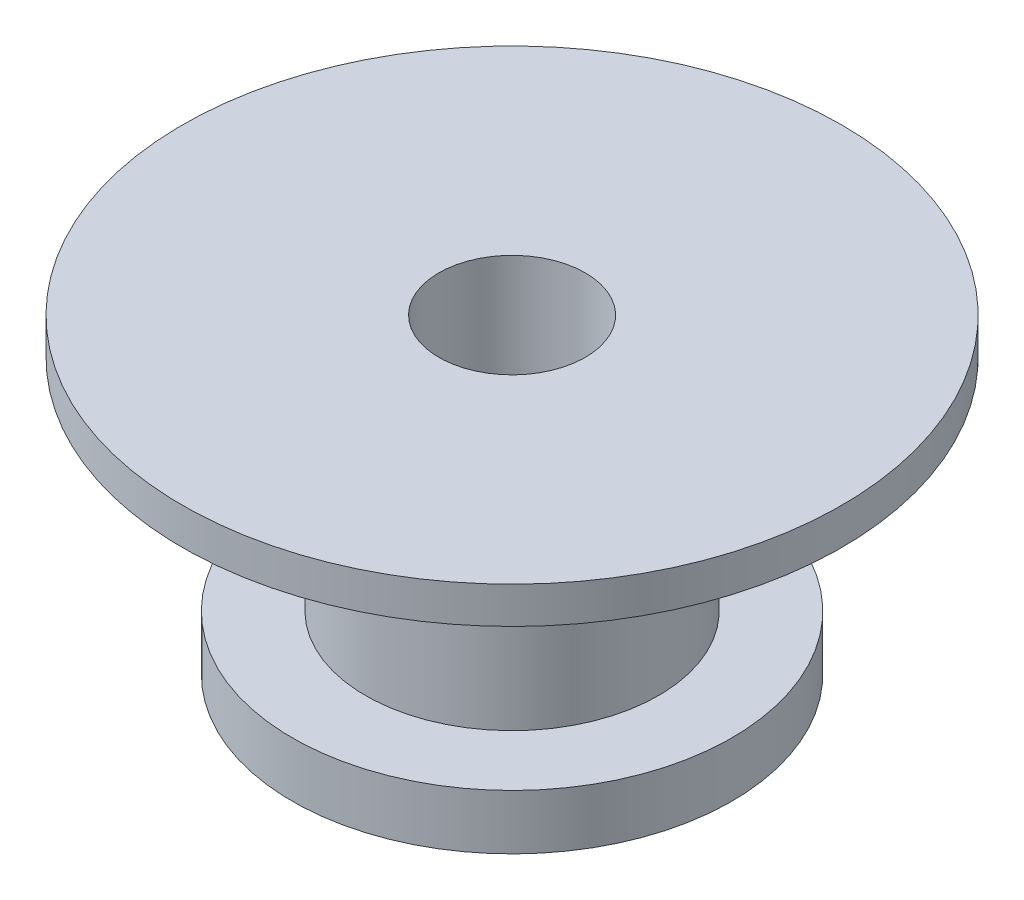
SolidWorks part; units mm, degrees
ref_plane "Front Plane" through (0, 0, 0) normal (0, 0, 1) x (1, 0, 0)
ref_plane "Top Plane" through (0, 0, 0) normal (0, 1, 0) x (1, 0, 0)
ref_plane "Right Plane" through (0, 0, 0) normal (1, 0, 0) x (0, 0, -1)
sketch "Sketch1" plane through (0, 0, 0) normal (0, 0, 1) x (1, 0, 0)
  line L0 (2, 7) -> (2, -1.5)
  line L4 (4, 0) -> (4, 6)
  line L5 (4, 6) -> (9, 6)
  line L7 (2, 7) -> (9, 7)
  line L8 (9, 6) -> (9, 7)
  line L9 (4, 0) -> (6, 0)
  line L11 (2, -1.5) -> (6, -1.5)
  line L12 (6, 0) -> (6, -1.5)
  line L13 (0, 0) -> (0, 8.3589) construction
  dimension "D1" = 6
  dimension "D2" = 8.5
  dimension "D3" = 2
  dimension "D4" = 1
  dimension "D5" = 9
  dimension "D6" = 4
  dimension "D7" = 6
revolve "Revolve1" add sketch "Sketch1" angle 360 about L13
